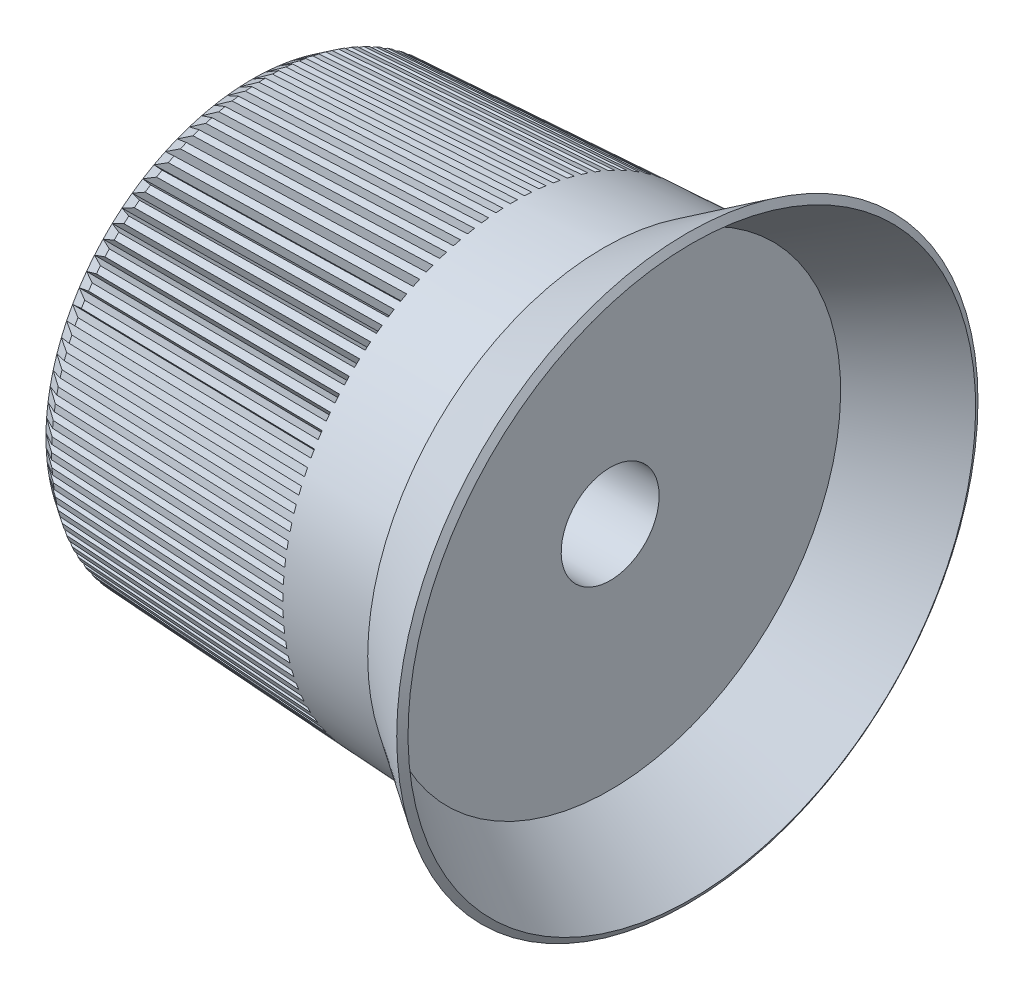
SolidWorks part; units mm, degrees
ref_plane "Front Plane" through (0, 0, 0) normal (0, 0, 1) x (1, 0, 0)
ref_plane "Top Plane" through (0, 0, 0) normal (0, 1, 0) x (1, 0, 0)
ref_plane "Right Plane" through (0, 0, 0) normal (1, 0, 0) x (0, 0, -1)
sketch "Sketch1" plane through (0, 0, 0) normal (0, 0, 1) x (1, 0, 0)
  line L0 (0, 0) -> (0, 26.5)
  line L1 (0, 26.5) -> (43, 28.9)
  line L2 (43, 28.9) -> (53.253, 35.6)
  line L3 (53.253, 35.6) -> (53.8, 34.7629)
  line L4 (53.8, 34.7629) -> (43.8, 28.2282)
  line L5 (43.8, 28.2282) -> (43.8, 6)
  line L6 (43.8, 6) -> (3.8, 6)
  line L7 (3.8, 6) -> (3.8, 0)
  line L8 (3.8, 0) -> (0, 0)
  dimension "D1" = 6
  dimension "D2" = 53.8
  dimension "D3" = 43
  dimension "D4" = 1
  dimension "D5" = 26.5
  dimension "D6" = 28.9
  dimension "D7" = 35.6
  dimension "D8" = 43.8
  dimension "D9" = 40
revolve "Revolve1" add sketch "Sketch1" angle 360 about L8
chamfer "Chamfer1" distance 2 angle 30 1 edges at (0, 26.5, 0)
sketch "Sketch2" plane through (0, 0, 0) normal (-1, 0, 0) x (0, 0, 1)
  line L0 (0, 25.305) -> (1.8199, 30.305)
  line L1 (1.8199, 30.305) -> (-1.8199, 30.305)
  line L2 (-1.8199, 30.305) -> (0, 25.305)
  line L3 (0, 25.305) -> (0, 30.305) construction
  circle A0 centre (0, 0) radius 25.305 construction
  dimension "D1" = 40
  dimension "D2" = 20
  dimension "D3" = 5
sketch "Sketch3" plane through (0, 0, 0) normal (0, 0, 1) x (1, 0, 0)
  line L0 (0, 25.305) -> (32, 27.091)
  line L1 (0, 25.305) -> (0, 30.305) construction
  line L2 (43, 28.9) -> (43, -28.9) construction
  line L3 (43, 28.9) -> (1.9969, 26.6115) construction
  dimension "D1" = 11
sweep "Cut-Sweep1" cut profiles "Sketch2" path "Sketch3"
pattern_circular "CirPattern1" count 101 over 360 about axis through (0, 0, 0) along (1, 0, 0) of "Cut-Sweep1"
sketch "Sketch4" plane through (0, 0, 0) normal (0, 1, 0) x (1, 0, 0)
  line L0 (53.8, 0) -> (25.8, 0) construction
  line L1 (53.8, -34.7629) -> (53.8, 34.7629) construction
  circle A0 centre (25.8, 0) radius 3
  dimension "D1" = 6
  dimension "D2" = 28
extrude "Cut-Extrude1" cut sketch "Sketch4" against normal blind 90
